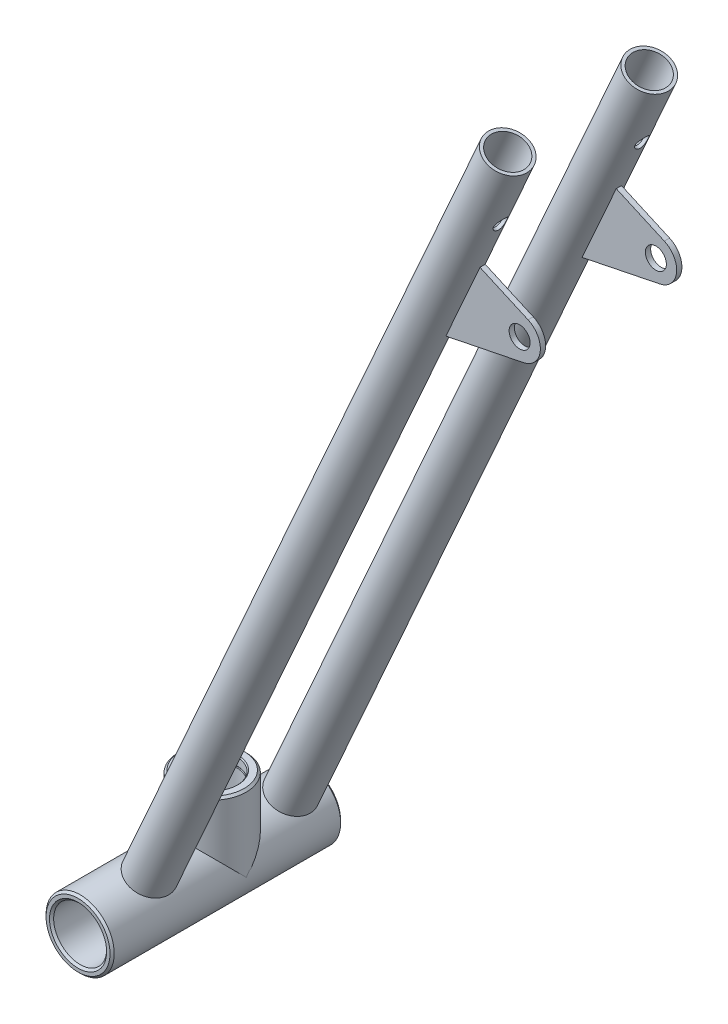
SolidWorks part; units mm, degrees
ref_plane "前视基准面" through (0, 0, 0) normal (0, 0, 1) x (1, 0, 0)
ref_plane "上视基准面" through (0, 0, 0) normal (0, 1, 0) x (1, 0, 0)
ref_plane "右视基准面" through (0, 0, 0) normal (1, 0, 0) x (0, 0, -1)
sketch "草图1" plane through (0, 0, 0) normal (0, 0, 1) x (1, 0, 0)
  circle A0 centre (0, 0) radius 32.5
  circle A1 centre (0, 0) radius 25.25
  dimension "D1" = 65
  dimension "D2" = 50.5
extrude "凸台-拉伸1" add sketch "草图1" along normal blind 220
ref_plane "基准面1" through (0, 72.5, 0) normal (0, 1, 0) x (1, 0, 0)
sketch "草图3" plane through (0, 72.5, 0) normal (0, 1, 0) x (1, 0, 0)
  circle A0 centre (0, -92) radius 32.5
  circle A1 centre (0, -92) radius 23.5
  dimension "D1" = 92
  dimension "D2" = 65
  dimension "D3" = 47
extrude "凸台-拉伸2" add sketch "草图3" against normal up to surface (40 mm away) separate body
sketch "草图4" plane through (0, 72.5, 0) normal (0, 1, 0) x (1, 0, 0)
  circle A0 centre (0, -92) radius 23.5
extrude "切除-拉伸2" cut sketch "草图4" against normal blind 70
chamfer "倒角1" distance 2 angle 45 1 edges at (0, 72.5, 124.5)
chamfer "倒角2" distance 2 angle 45 2 edges at (32.5, 0, 0) (32.5, 0, 220)
chamfer "倒角3" distance 1 angle 45 1 edges at (0, 72.5, 115.5)
ref_plane "基准面2" through (0, 62.5, 0) normal (0, 1, 0) x (1, 0, 0)
sketch "草图5" plane through (0, 62.5, 0) normal (0, 1, 0) x (1, 0, 0)
  circle A0 centre (0, -92) radius 24.75
  dimension "D1" = 49.5
extrude "切除-拉伸3" cut sketch "草图5" along normal blind 1.7
chamfer "倒角4" distance 2 angle 45 2 edges at (25.25, 0, 220) (25.25, 0, 0)
ref_plane "基准面3" through (0, 0, 10) normal (0, 0, -1) x (-1, 0, 0)
sketch "草图6" plane through (0, 0, 10) normal (0, 0, -1) x (-1, 0, 0)
  line L1 (0, 32.5) -> (0, 227.5172) construction
  line L2 (-13.2189, 29.6902) -> (-354.8777, 797.0684)
  arc A0 (32.5, 0) -> (-32.5, 0) centre (0, 0) ccw construction
  circle A1 centre (0, 0) radius 32.5 construction
  dimension "D1" = 24
  dimension "D2" = 840
other "冷弯空心圆管gb∕t6728-2002 42.3 X 3(1)"
ref_plane "基准面8" through (13.2189, 29.6902, 30) normal (0.4067, 0.9135, 0) x (0.9135, -0.4067, 0)
sketch "Sketch1" plane through (13.2189, 29.6902, 30) normal (0.4067, 0.9135, 0) x (0.9135, -0.4067, 0)
  line L0 (0, 0) -> (0, 20) construction
  circle A0 centre (0, 0) radius 17
  circle A1 centre (0, 0) radius 20
  point P3 (0, 0)
  dimension "Out_dia" = 40
  dimension "D1" = 3
  dimension "D2" = 34
ref_plane "基准面9" through (0, 0, 0) normal (0.9135, -0.4067, 0) x (0.4067, 0.9135, 0)
sketch "草图7" plane through (0, 0, 0) normal (0.9135, -0.4067, 0) x (0.4067, 0.9135, 0)
  line L1 (872.5, 30) -> (722.3924, 30) construction
  line L3 (872.5, 10) -> (872.5, 50) construction
  circle A0 centre (812.5, 30) radius 6.5
  dimension "D2" = 13
  dimension "D1" = 60
ref_plane "基准面10" through (0, 0, 97.5) normal (0, 0, -1) x (-1, 0, 0)
extrude "切除-拉伸6" cut sketch "草图7" against normal mid plane 50
ref_plane "基准面11" through (0, 0, 30) normal (0, 0, -1) x (-1, 0, 0)
sketch "草图8" plane through (0, 0, 30) normal (0, 0, -1) x (-1, 0, 0)
  line L0 (-328.4076, 688.4437) -> (-295.8687, 615.36)
  line L1 (-346.1006, 728.1829) -> (-31.4899, 21.5555) construction
  line L2 (-328.4076, 688.4437) -> (-374.2612, 668.0283)
  line L5 (-370.1666, 630.527) -> (-295.8687, 615.36)
  arc A1 (-374.2612, 668.0283) -> (-370.1666, 630.527) centre (-366.205, 649.9338) ccw
  circle A2 centre (-366.205, 649.9338) radius 10
  dimension "D4" = 19.807
  dimension "D5" = 20
  dimension "D1" = 110
  dimension "D2" = 80
  dimension "D3" = 75.8302
extrude "凸台-拉伸3" add sketch "草图8" against normal blind 5 separate body
mirror "镜向3" about plane through (0, 0, 97.5) normal (0, 0, -1) of bodies 118 120
